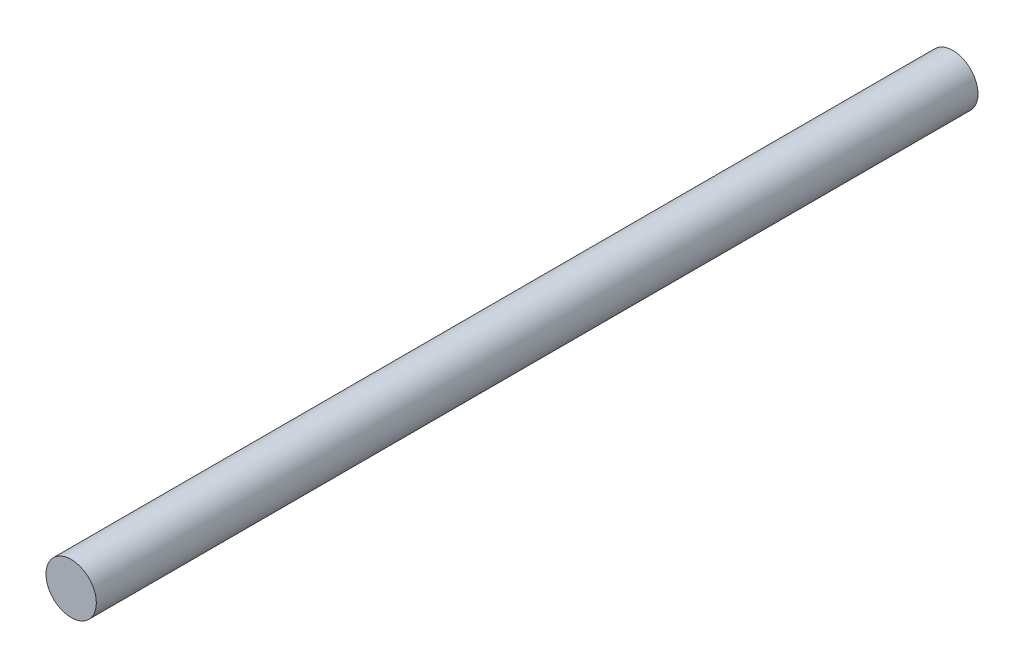
from build123d import *

# Parameters (mm, degrees)
SKETCH_1_R      = 4
EXTRUDE_1_DEPTH = 70


with BuildPart() as part:
    # 草图1 → 凸台-拉伸1 (new, symmetric)
    with BuildSketch(Plane.XY):
        Circle(SKETCH_1_R)
    extrude(amount=EXTRUDE_1_DEPTH, both=True)


solid = part.part
